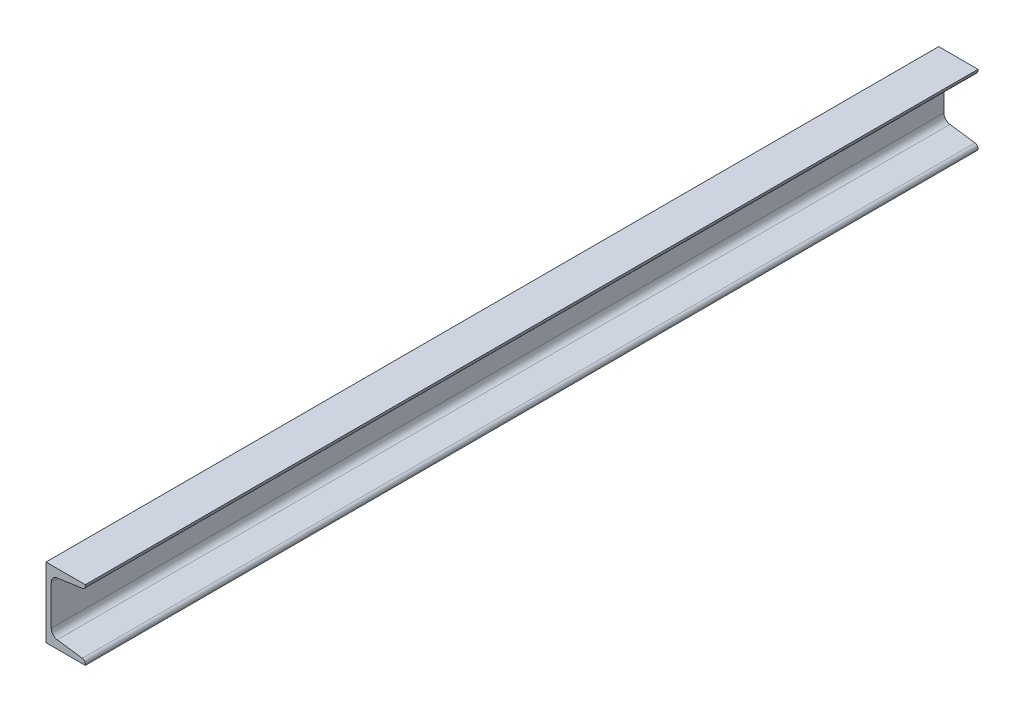
from build123d import *

# Parameters (mm, degrees)
BOSS_EXTRUDE1_DEPTH = 1022


with BuildPart() as part:
    # Sketch1 → Boss-Extrude1 (new body)
    with BuildSketch(Plane.XY):
        with BuildLine():
            Line((0, 0), (-45, 0))
            Line((-45, 0), (-45, -80))
            Line((-45, -80), (0, -80))
            Line((0, -80), (0, -78.639315732))
            ThreePointArc((0, -78.639315732), (-0.981161679, -76.015079616), (-3.443307596, -74.678243457))
            Line((-3.443307596, -74.678243457), (-32.113384808, -70.648926875))
            ThreePointArc((-32.113384808, -70.648926875), (-37.037676642, -67.975254557), (-39, -62.726782325))
            Line((-39, -62.726782325), (-39, -17.273217675))
            ThreePointArc((-39, -17.273217675), (-37.037676642, -12.024745443), (-32.113384808, -9.351073125))
            Line((-32.113384808, -9.351073125), (-3.443307596, -5.321756543))
            ThreePointArc((-3.443307596, -5.321756543), (-0.981161679, -3.984920384), (0, -1.360684268))
            Line((0, -1.360684268), (0, 0))
        make_face()
    extrude(amount=BOSS_EXTRUDE1_DEPTH)


solid = part.part
